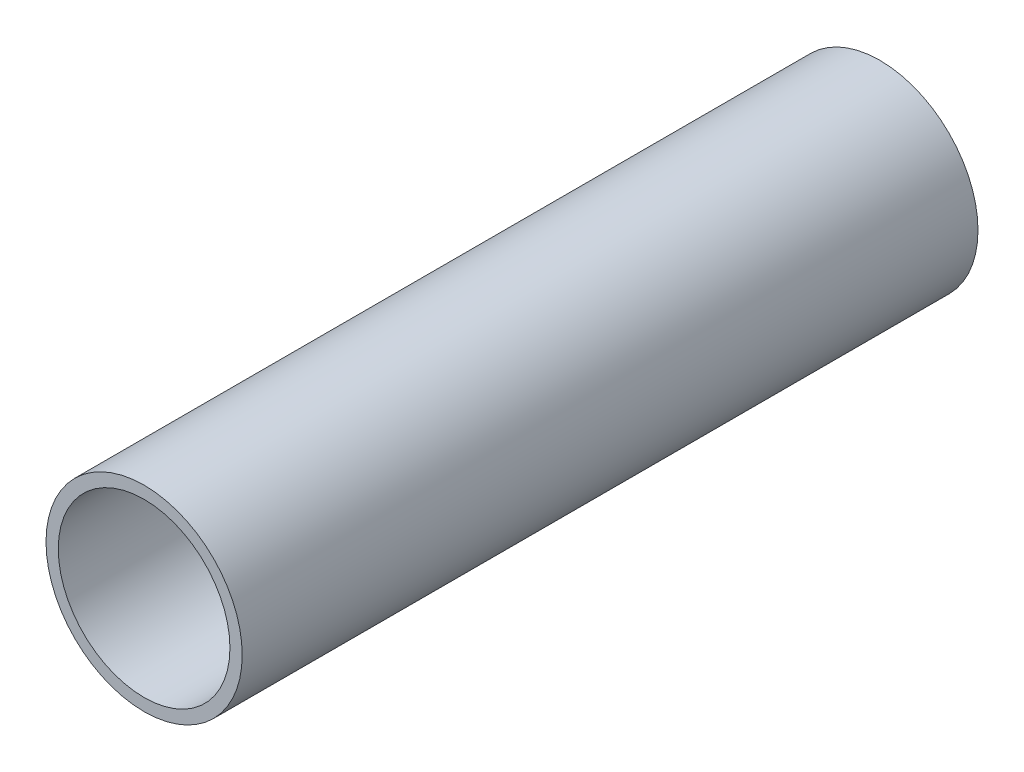
from build123d import *

# Parameters (mm, degrees)
SKETCH1_R           = 14.4
SKETCH1_R_2         = 12.6
BOSS_EXTRUDE1_DEPTH = 108


with BuildPart() as part:
    # Sketch1 → Boss-Extrude1 (new body)
    with BuildSketch(Plane.XY):
        Circle(SKETCH1_R)
        Circle(SKETCH1_R_2, mode=Mode.SUBTRACT)
    extrude(amount=BOSS_EXTRUDE1_DEPTH)


solid = part.part
